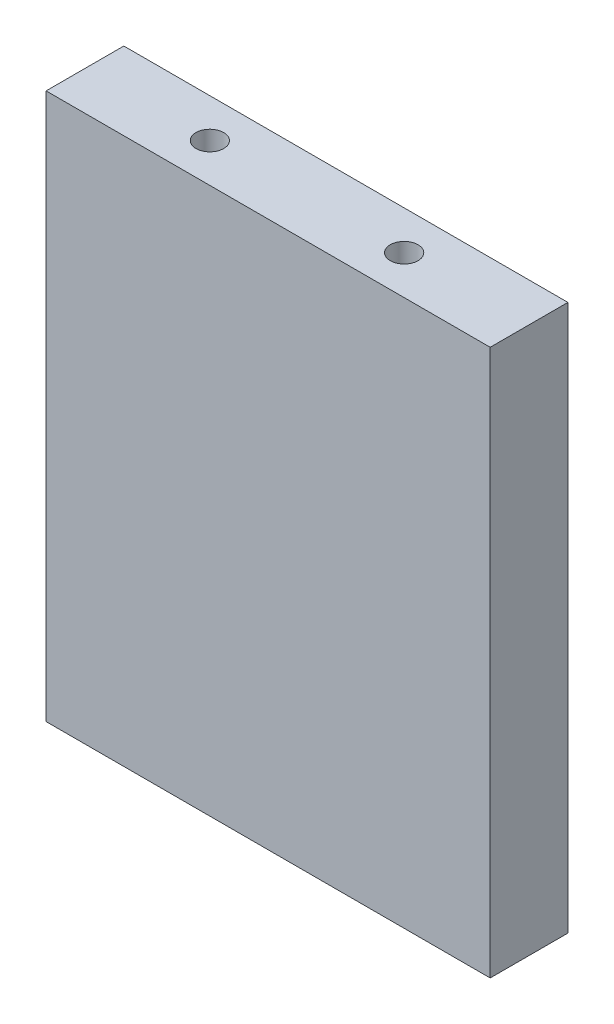
from build123d import *

# Parameters (mm, degrees)
SKETCH_1_W             = 80
SKETCH_1_H             = 98.4
EXTRUDE_1_DEPTH        = 14
HOLE_WIZARD_M6_1_D     = 5
HOLE_WIZARD_M6_1_DEPTH = 17
HOLE_WIZARD_M6_1_TIP   = 1.502151548
HOLE_WIZARD_M6_2_D     = 5
HOLE_WIZARD_M6_2_DEPTH = 17
HOLE_WIZARD_M6_2_TIP   = 1.502151548


with BuildPart() as part:
    # 草图1 → 凸台-拉伸1 (new body)
    with BuildSketch(Plane.XY):
        Rectangle(SKETCH_1_W, SKETCH_1_H)
    extrude(amount=EXTRUDE_1_DEPTH)

    # M6 螺纹孔1
    with Locations(Plane(origin=(0, -49.2, 0), x_dir=(-1, 0, 0), z_dir=(0, -1, 0))):
        with Locations((-21, -7), (21, -7)):
            Hole(HOLE_WIZARD_M6_1_D / 2, depth=HOLE_WIZARD_M6_1_DEPTH)
            with Locations((0, 0, -(HOLE_WIZARD_M6_1_DEPTH + HOLE_WIZARD_M6_1_TIP / 2))):  # 118° drill point
                Cone(0, HOLE_WIZARD_M6_1_D / 2, HOLE_WIZARD_M6_1_TIP, mode=Mode.SUBTRACT)

    # M6 螺纹孔2
    with Locations(Plane(origin=(0, 49.2, 0), x_dir=(1, 0, 0), z_dir=(0, 1, 0))):
        with Locations((-17.5, -7), (17.5, -7)):
            Hole(HOLE_WIZARD_M6_2_D / 2, depth=HOLE_WIZARD_M6_2_DEPTH)
            with Locations((0, 0, -(HOLE_WIZARD_M6_2_DEPTH + HOLE_WIZARD_M6_2_TIP / 2))):  # 118° drill point
                Cone(0, HOLE_WIZARD_M6_2_D / 2, HOLE_WIZARD_M6_2_TIP, mode=Mode.SUBTRACT)


solid = part.part
